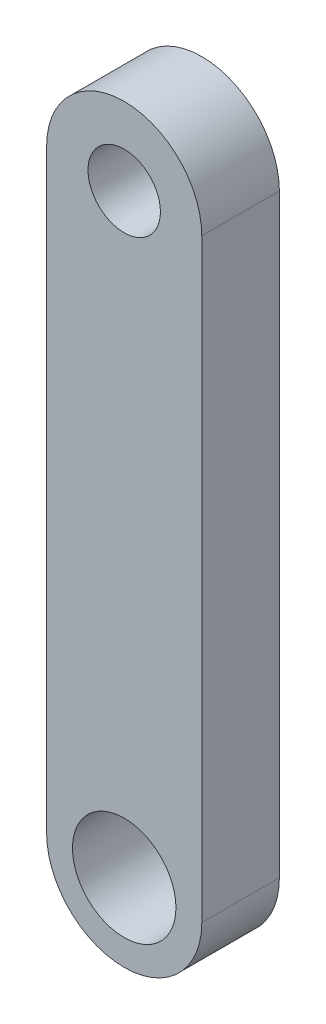
from build123d import *

# Parameters (mm, degrees)
EXTRUDE_1_DEPTH     = 15
SKETCH_2_R          = 7
SKETCH_2_R_2        = 10
CUT_EXTRUDE_1_DEPTH = 132.719398723


with BuildPart() as part:
    # 草图1 → 凸台-拉伸1 (new body)
    with BuildSketch(Plane.XY):
        with BuildLine():
            Line((-15, 0), (-15, 115))
            ThreePointArc((-15, 115), (0, 130), (15, 115))
            Line((15, 115), (15, 0))
            ThreePointArc((15, 0), (0, -15), (-15, 0))
        make_face()
    extrude(amount=EXTRUDE_1_DEPTH)

    # 草图2 → 切除-拉伸1 (cut, through all)
    with BuildSketch(Plane.XY.offset(15)):
        with Locations((0, 115)):
            Circle(SKETCH_2_R)
        Circle(SKETCH_2_R_2)
    extrude(amount=-CUT_EXTRUDE_1_DEPTH, mode=Mode.SUBTRACT)


solid = part.part
